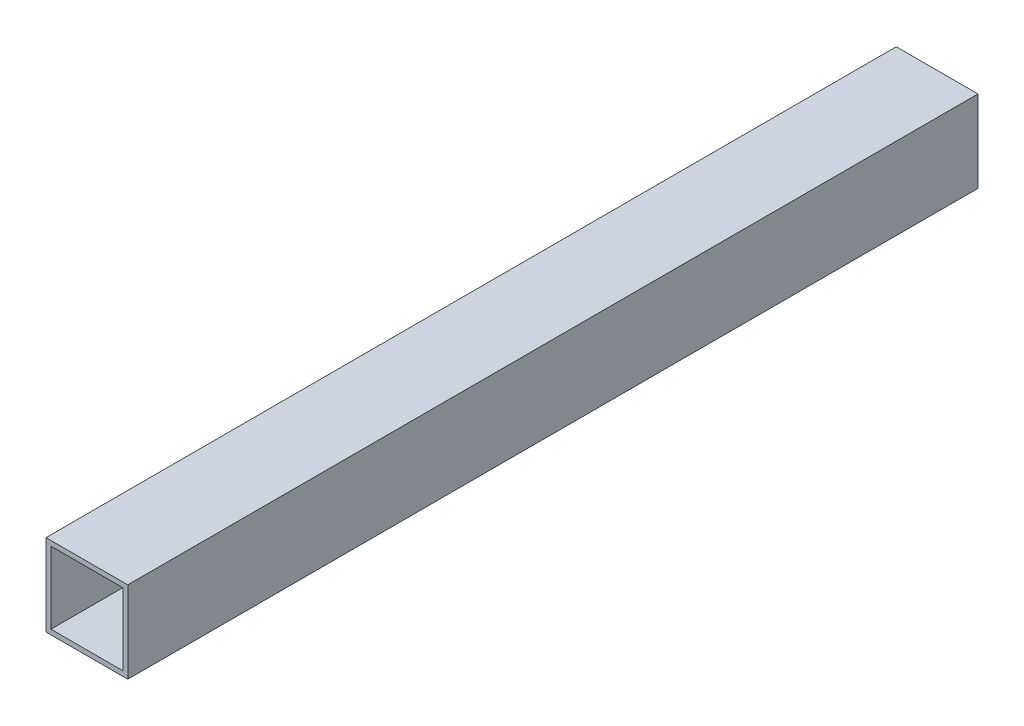
from build123d import *

# Parameters (mm, degrees)
SKETCH_1_W      = 50
SKETCH_1_H      = 50
SKETCH_1_W_2    = 44
SKETCH_1_H_2    = 44
EXTRUDE_1_DEPTH = 520


with BuildPart() as part:
    # 草图1 → 凸台-拉伸1 (new body)
    with BuildSketch(Plane.XY):
        with Locations((25, 25)):
            Rectangle(SKETCH_1_W, SKETCH_1_H)
        with Locations((25, 25)):
            Rectangle(SKETCH_1_W_2, SKETCH_1_H_2, mode=Mode.SUBTRACT)
    extrude(amount=EXTRUDE_1_DEPTH)


solid = part.part
